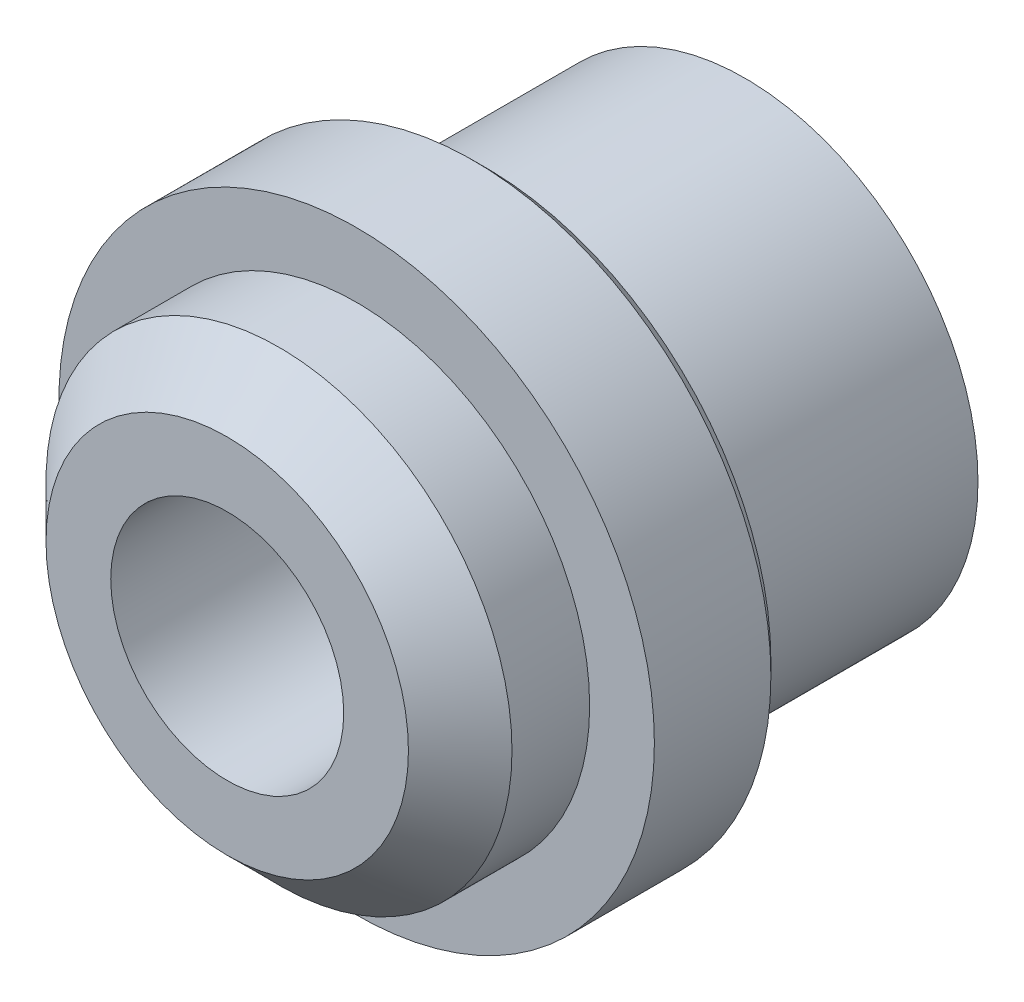
SolidWorks part; units mm, degrees
ref_plane "Front Plane" through (0, 0, 0) normal (0, 0, 1) x (1, 0, 0)
ref_plane "Top Plane" through (0, 0, 0) normal (0, 1, 0) x (1, 0, 0)
ref_plane "Right Plane" through (0, 0, 0) normal (1, 0, 0) x (0, 0, -1)
sketch "Sketch1" plane through (0, 0, 0) normal (0, 0, 1) x (1, 0, 0)
  circle A0 centre (0, 0) radius 18
  dimension "D1" = 36
extrude "Boss-Extrude1" add sketch "Sketch1" along normal blind 20
sketch "Sketch2" plane through (0, 0, 20) normal (0, 0, 1) x (1, 0, 0)
  circle A0 centre (0, 0) radius 23
  dimension "D1" = 46
extrude "Boss-Extrude2" add sketch "Sketch2" along normal blind 10
sketch "Sketch3" plane through (0, 0, 30) normal (0, 0, 1) x (1, 0, 0)
  circle A0 centre (0, 0) radius 18
  dimension "D1" = 36
extrude "Boss-Extrude3" add sketch "Sketch3" along normal blind 10
chamfer "Chamfer1" distance 4 angle 45 1 edges at (18, 0, 40)
sketch "Sketch4" plane through (0, 0, 40) normal (0, 0, 1) x (1, 0, 0)
  circle A0 centre (0, 0) radius 9
  dimension "D1" = 18
extrude "Cut-Extrude1" cut sketch "Sketch4" against normal through all
chamfer "Chamfer2" distance 1 angle 45 1 edges at (23, 0, 20)
